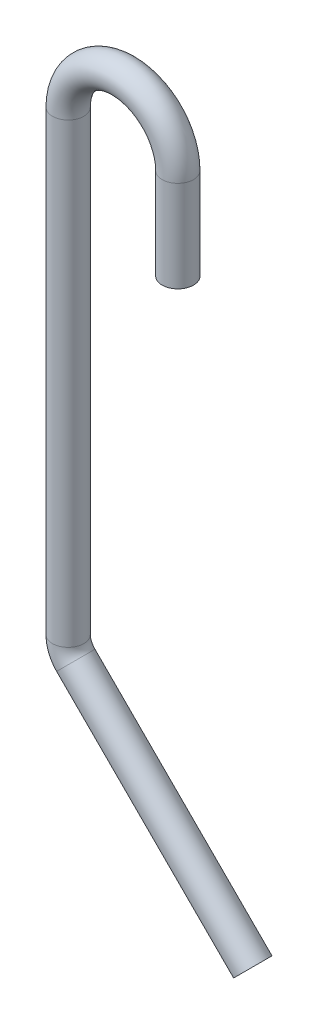
SolidWorks part; units mm, degrees
material "A3"
ref_plane "前视基准面" through (0, 0, 0) normal (0, 0, 1) x (1, 0, 0)
ref_plane "上视基准面" through (0, 0, 0) normal (0, 1, 0) x (1, 0, 0)
ref_plane "右视基准面" through (0, 0, 0) normal (1, 0, 0) x (0, 0, -1)
sketch "草图1" plane through (0, 0, 0) normal (0, 0, 1) x (1, 0, 0)
  line L0 (0, 0) -> (-67.7817, 67.7817)
  line L1 (-70.7107, 74.8528) -> (-70.7107, 249.7107)
  line L2 (-28.7107, 249.7107) -> (-28.7107, 214.7107)
  arc A0 (-70.7107, 249.7107) -> (-28.7107, 249.7107) centre (-49.7107, 249.7107) cw
  arc A1 (-67.7817, 67.7817) -> (-70.7107, 74.8528) centre (-60.7107, 74.8528) cw
  point P6 (-49.7107, 270.7107)
  point P10 (-70.7107, 70.7107)
  dimension "D1" = 100
  dimension "D5" = 21
  dimension "D6" = 10
  dimension "D2" = 200
  dimension "D3" = 45
  dimension "D4" = 35
sweep "扫描1" add path "草图1" circular profile diameter 12 parameters "D3"=12
